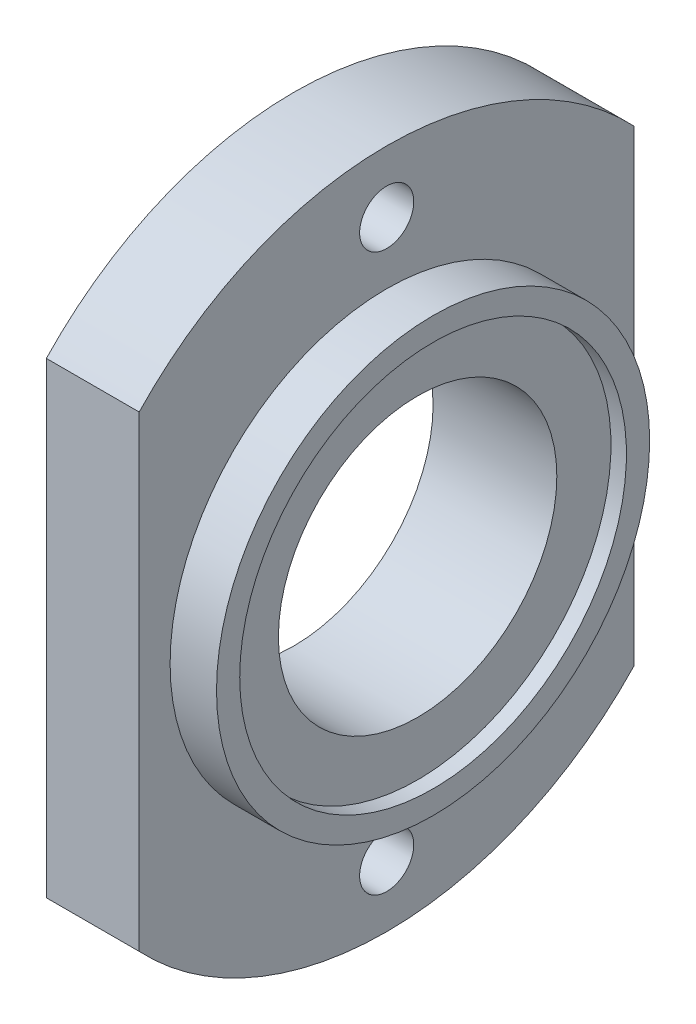
SolidWorks part; units mm, degrees
ref_plane "Front Plane" through (0, 0, 0) normal (0, 0, 1) x (1, 0, 0)
ref_plane "Top Plane" through (0, 0, 0) normal (0, 1, 0) x (1, 0, 0)
ref_plane "Right Plane" through (0, 0, 0) normal (1, 0, 0) x (0, 0, -1)
sketch "Sketch1" plane through (0, 0, 0) normal (0, 0, 1) x (1, 0, 0)
  line L0 (0, 9) -> (0, 22)
  line L1 (0, 22) -> (6, 22)
  line L2 (6, 22) -> (6, 14)
  line L3 (6, 14) -> (9, 14)
  line L4 (9, 14) -> (9, 12.5)
  line L5 (9, 12.5) -> (8, 12.5)
  line L6 (8, 12.5) -> (8, 9)
  line L7 (8, 9) -> (0, 9)
  line L8 (0, 0) -> (35.7199, 0) construction
  dimension "D1" = 22
  dimension "D2" = 9
  dimension "D3" = 9
  dimension "D4" = 3
  dimension "D5" = 1
  dimension "D6" = 12.5
  dimension "D7" = 14
revolve "Revolve1" add sketch "Sketch1" angle 360 about L8
sketch "Sketch3" plane through (0, 0, 0) normal (-1, 0, 0) x (0, 0, 1)
  line L1 (-16, 25) -> (16, 25)
  line L2 (-16, 25) -> (-16, -25)
  line L3 (-16, -25) -> (16, -25)
  line L4 (16, 25) -> (16, -25)
  line L5 (-16, 25) -> (16, -25) construction
  line L6 (-16, -25) -> (16, 25) construction
  point P0 (0, 0)
  dimension "D1" = 32
  dimension "D2" = 50
extrude "Cut-Extrude1" cut sketch "Sketch3" against normal through all flip side to cut
hole_wizard "CBORE for M3 Hex Head Bolt1" positions "Sketch5" profile "Sketch4" counterbore size "M3" standard "GB" end condition through all
sketch "Sketch5" plane through (0, 0, 0) normal (-1, 0, 0) x (0, 0, 1)
  line L0 (-16, 0) -> (16, 0) construction
  line L1 (-16, 15.0997) -> (-16, -15.0997) construction
  line L2 (16, -15.0997) -> (16, 15.0997) construction
  point P0 (0, 18)
  point P1 (0, -18)
  dimension "D1" = 36
sketch "Sketch4" plane through (0, 18, 0) normal (0, 1, 0) x (0, 0, 1)
  line L0 (0, 0) -> (0, 9)
  line L1 (0, 9) -> (1.75, 9)
  line L3 (1.75, 9) -> (1.75, 3.5)
  line L4 (1.75, 3.5) -> (3, 3.5)
  line L5 (3, 3.5) -> (3, 0)
  line L7 (3, 0) -> (0, 0)
  line L11 (0, -6.35) -> (0, 107.95) construction
  dimension "通孔孔直径" = 3.5
  dimension "通孔孔深度" = 9
  dimension "柱形沉头孔直径" = 6
  dimension "柱形沉头孔深度" = 3.5
